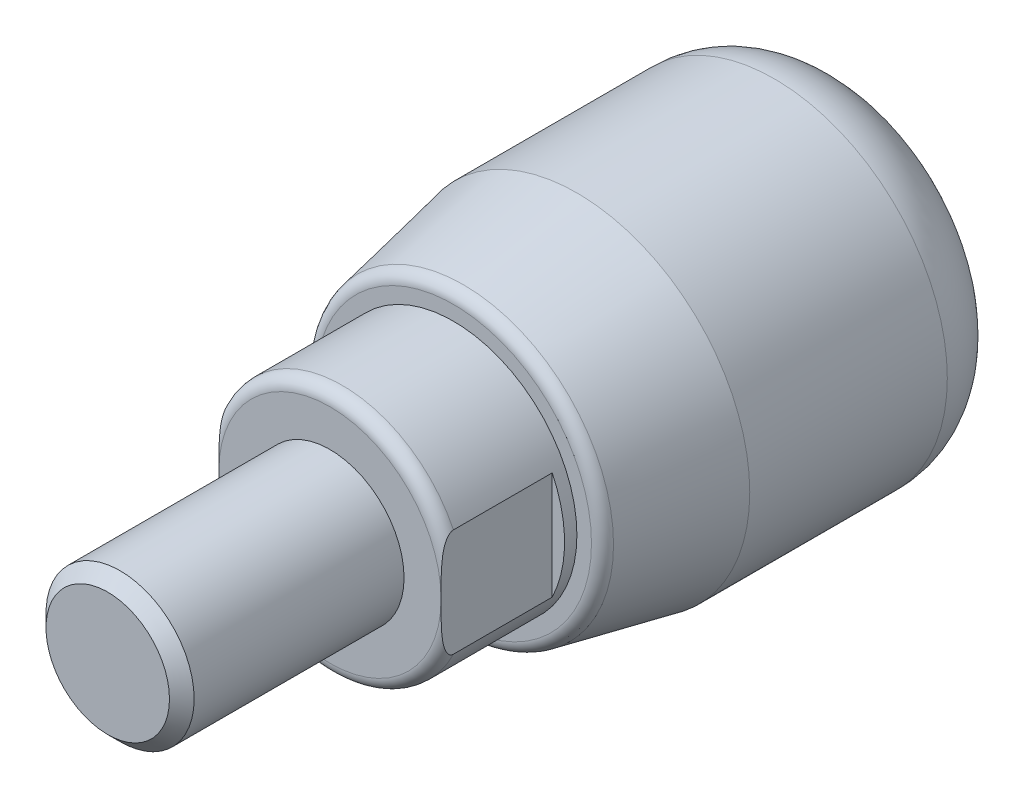
from build123d import *

# Parameters (mm, degrees)
SKETCH1_R           = 7
BOSS_EXTRUDE1_DEPTH = 8
SKETCH2_R           = 5
BOSS_EXTRUDE2_DEPTH = 5
SKETCH3_R           = 3
BOSS_EXTRUDE3_DEPTH = 9
CHAMFER1_SIZE       = 5
CHAMFER1_SIZE2      = 1
FILLET1_R           = 3
FILLET2_R           = 0.5
FILLET3_R           = 0.5
SKETCH4_OUTSIDE_W   = 23.188
SKETCH4_OUTSIDE_H   = 23.188
SKETCH4_OUTSIDE_W_2 = 9
SKETCH4_OUTSIDE_H_2 = 10
CUT_EXTRUDE1_DEPTH  = 4.5
CHAMFER3_SIZE       = 0.5


with BuildPart() as part:
    # Sketch1 → Boss-Extrude1 (new, symmetric)
    with BuildSketch(Plane.XY):
        Circle(SKETCH1_R)
    extrude(amount=BOSS_EXTRUDE1_DEPTH, both=True)

    # Sketch2 → Boss-Extrude2 (add)
    with BuildSketch(Plane.XY.offset(8)):
        Circle(SKETCH2_R)
    extrude(amount=BOSS_EXTRUDE2_DEPTH)

    # Sketch3 → Boss-Extrude3 (add)
    with BuildSketch(Plane.XY.offset(13)):
        Circle(SKETCH3_R)
    extrude(amount=BOSS_EXTRUDE3_DEPTH)

    # Chamfer1
    chamfer1_edges = [part.edges().sort_by_distance(p)[0] for p in [
        (-7, 0, 8),
    ]]
    chamfer1_side = [part.faces().sort_by_distance(p)[0] for p in [
        (-7, 0, 0),
    ]]
    chamfer(chamfer1_edges, length=CHAMFER1_SIZE, length2=CHAMFER1_SIZE2, reference=chamfer1_side[0])

    # Fillet1
    fillet1_edges = [part.edges().sort_by_distance(p)[0] for p in [
        (-7, 0, -8),
    ]]
    fillet(fillet1_edges, radius=FILLET1_R)

    # Fillet2
    fillet2_edges = [part.edges().sort_by_distance(p)[0] for p in [
        (-6, 0, 8),
    ]]
    fillet(fillet2_edges, radius=FILLET2_R)

    # Fillet3
    fillet3_edges = [part.edges().sort_by_distance(p)[0] for p in [
        (-5, 0, 13),
    ]]
    fillet(fillet3_edges, radius=FILLET3_R)

    # Sketch4 outside → Cut-Extrude1 (cut)
    with BuildSketch(Plane.XY.offset(13)):
        Rectangle(SKETCH4_OUTSIDE_W, SKETCH4_OUTSIDE_H)
        Rectangle(SKETCH4_OUTSIDE_W_2, SKETCH4_OUTSIDE_H_2, mode=Mode.SUBTRACT)
    extrude(amount=-CUT_EXTRUDE1_DEPTH, mode=Mode.SUBTRACT)

    # Chamfer3
    chamfer3_edges = [part.edges().sort_by_distance(p)[0] for p in [
        (-3, 0, 22),
    ]]
    chamfer(chamfer3_edges, length=CHAMFER3_SIZE)


solid = part.part
